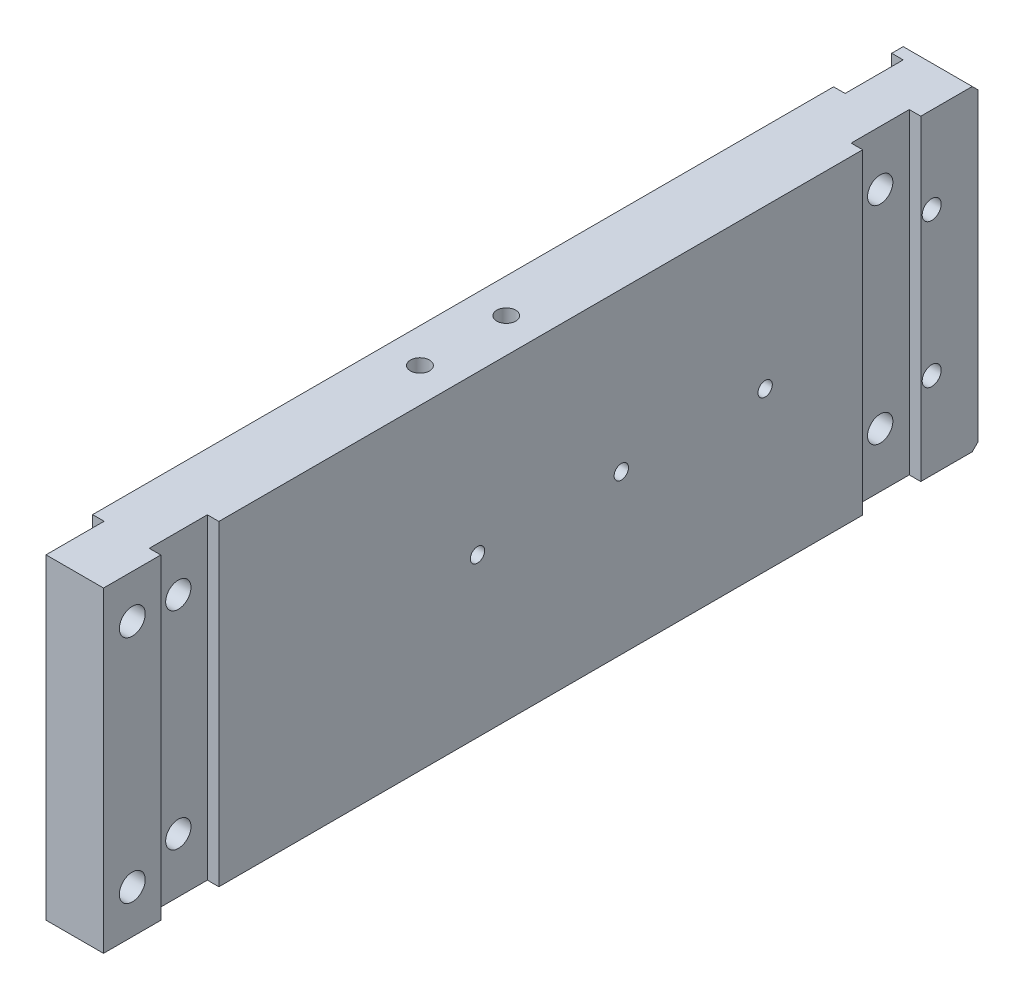
SolidWorks part; units mm, degrees
material "6061铝"
ref_plane "前视基准面" through (0, 0, 0) normal (0, 0, 1) x (1, 0, 0)
ref_plane "上视基准面" through (0, 0, 0) normal (0, 1, 0) x (1, 0, 0)
ref_plane "右视基准面" through (0, 0, 0) normal (1, 0, 0) x (0, 0, -1)
sketch "草图1" plane through (0, 0, 0) normal (1, 0, 0) x (0, 0, -1)
  line L1 (-76, 27.5) -> (76, 27.5)
  line L2 (-76, 27.5) -> (-76, -27.5)
  line L3 (-76, -27.5) -> (76, -27.5)
  line L4 (76, 27.5) -> (76, -27.5)
  line L5 (-76, 27.5) -> (76, -27.5) construction
  line L6 (-76, -27.5) -> (76, 27.5) construction
  point P0 (0, 0)
  dimension "D1" = 55
  dimension "D2" = 152
extrude "凸台-拉伸1" add sketch "草图1" along normal blind 12
sketch "草图2" plane through (12, 0, 0) normal (1, 0, 0) x (0, 0, -1)
  line L0 (-76, 27.5) -> (-76, -27.5) construction
  line L1 (-66.05, 33.3411) -> (-55.95, 33.3411)
  line L2 (-66.05, 33.3411) -> (-66.05, -34.4007)
  line L3 (-66.05, -34.4007) -> (-55.95, -34.4007)
  line L4 (-55.95, 33.3411) -> (-55.95, -34.4007)
  line L5 (-66.05, 33.3411) -> (-55.95, -34.4007) construction
  line L6 (-66.05, -34.4007) -> (-55.95, 33.3411) construction
  point P0 (-61, -0.5298)
  dimension "D1" = 10.1
  dimension "D2" = 15
extrude "切除-拉伸1" cut sketch "草图2" against normal blind 2
sketch "草图3" plane through (0, 0, 0) normal (-1, 0, 0) x (0, 0, 1)
  line L0 (0, 0) -> (-87.8664, 0) construction
  line L2 (-54, 6.025) -> (27, 6.025)
  line L3 (-54, 6.025) -> (-54, -6.025)
  line L4 (-54, -6.025) -> (27, -6.025)
  line L5 (27, 6.025) -> (27, -6.025)
  line L6 (-54, 6.025) -> (27, -6.025) construction
  line L7 (-54, -6.025) -> (27, 6.025) construction
  line L8 (76, 27.5) -> (76, -27.5) construction
  point P2 (-13.5, 0)
  dimension "D1" = 12.05
  dimension "D2" = 81
  dimension "D3" = 49
extrude "切除-拉伸2" cut sketch "草图3" against normal blind 1.5
sketch "草图4" plane through (0, 0, 0) normal (-1, 0, 0) x (0, 0, 1)
  circle A0 centre (-54, 6.025) radius 2
  circle A1 centre (-54, -6.025) radius 2
  circle A2 centre (27, -6.025) radius 2
  circle A3 centre (27, 6.025) radius 2
  dimension "D1" = 4
extrude "切除-拉伸3" cut sketch "草图4" against normal up to surface (1.5 mm away) up to face at (1.5, 0, -13.5)
sketch "草图5" plane through (0, -27.5, 0) normal (0, -1, 0) x (1, 0, 0)
  line L2 (0, 76) -> (2, 76)
  line L3 (0, 76) -> (0, 65.9)
  line L4 (0, 65.9) -> (2, 65.9)
  line L6 (2, 76) -> (2, 65.9)
  dimension "D1" = 2
  dimension "D2" = 10.1
extrude "切除-拉伸4" cut sketch "草图5" against normal blind 110
sketch "草图7" plane through (0, 27.5, 0) normal (0, 1, 0) x (1, 0, 0)
  line L0 (0, 76) -> (0, -65.9) construction
  line L1 (-2, 73) -> (2, 73)
  line L2 (-2, 73) -> (-2, 62.9)
  line L3 (-2, 62.9) -> (2, 62.9)
  line L4 (2, 73) -> (2, 62.9)
  line L5 (-2, 73) -> (2, 62.9) construction
  line L6 (-2, 62.9) -> (2, 73) construction
  line L7 (12, 76) -> (0, 76) construction
  point P0 (0, 67.95)
  dimension "D1" = 10.1
  dimension "D2" = 3
  dimension "D3" = 4
extrude "切除-拉伸5" cut sketch "草图7" against normal blind 120
chamfer "倒角1" distance 1 angle 45 2 edges at (6, -27.5, -76) (6, 27.5, -76)
hole_wizard "M4 螺纹孔1" positions "草图8" profile "草图9" tap size "M4" standard "GB"
sketch "草图8" plane through (0, 27.5, 0) normal (0, 1, 0) x (1, 0, 0)
  line L1 (12, -76) -> (2, -76) construction
  line L2 (12, 75) -> (12, -55.95) construction
  point P0 (6, -15)
  point P2 (6, 0)
  dimension "D1" = 15
  dimension "D2" = 61
  dimension "D3" = 6
cosmetic thread "孔螺蚊线1" parameters "D1"=6, "D2"=4
cosmetic thread "孔螺蚊线2" parameters "D1"=6, "D2"=4
sketch "草图9" plane through (6, 27.5, 15) normal (1, 0, 0) x (0, 0, 1)
  line L0 (0, 0) -> (0, 11.0914)
  line L1 (0, 11.0914) -> (1.65, 10.1)
  line L2 (1.65, 10.1) -> (1.65, 0)
  line L5 (1.65, 0) -> (0, 0)
  line L10 (0, 11.0914) -> (-1.65, 10.1) construction
  line L11 (0, -6.35) -> (0, 107.95) construction
  dimension "螺纹孔钻头直径" = 3.3
  dimension "螺纹孔钻头深度" = 10.1
  dimension "导头角度" = 118
mirror "镜向1" about plane through (0, 0, 0) normal (0, 1, 0) of "M4 螺纹孔1"
hole_wizard "Ø5.0 (5) 直径孔2" positions "草图16" profile "草图17" hole size "Ø5.0" standard "GB"
sketch "草图16" plane through (2, 0, 0) normal (-1, 0, 0) x (0, 0, 1)
  line L0 (0, 0) -> (90.5558, 0) construction
  line L2 (65.9, -27.5) -> (65.9, 27.5) construction
  point P0 (70.9, 12.5)
  point P8 (70.9, -12.5)
  dimension "D1" = 5
  dimension "D2" = 25
sketch "草图17" plane through (2, 12.5, 70.9) normal (0, 1, 0) x (0, 0, 1)
  line L0 (0, 0) -> (0, 7.5022)
  line L1 (0, 7.5022) -> (2.5, 6)
  line L2 (2.5, 6) -> (2.5, 0)
  line L5 (2.5, 0) -> (0, 0)
  line L10 (0, 7.5022) -> (-2.5, 6) construction
  line L11 (0, -6.35) -> (0, 107.95) construction
  dimension "孔直径" = 5
  dimension "孔深度" = 6
  dimension "导头角度" = 118
mirror "镜向2" about plane through (0, 0, 0) normal (0, 0, 1) of "切除-拉伸1"
hole_wizard "打孔尺寸(%根据)内六角圆柱头螺钉的类型1" positions "草图18" profile "草图19" counterbore size "M4" standard "GB" end condition through all
sketch "草图18" plane through (0, 0, 0) normal (-1, 0, 0) x (0, 0, 1)
  point P0 (61, -18)
  point P2 (61, 18)
  point P4 (-61, 18)
  point P6 (-61, -18)
sketch "草图19" plane through (0, -18, 61) normal (0, 1, 0) x (0, 0, 1)
  line L0 (0, 0) -> (0, 12)
  line L1 (0, 12) -> (2.2, 12)
  line L3 (2.2, 12) -> (2.2, 6)
  line L4 (2.2, 6) -> (4, 6)
  line L5 (4, 6) -> (4, 0)
  line L7 (4, 0) -> (0, 0)
  line L11 (0, -6.35) -> (0, 107.95) construction
  dimension "通孔孔直径" = 4.4
  dimension "通孔孔深度" = 12
  dimension "柱形沉头孔直径" = 8
  dimension "柱形沉头孔深度" = 6
hole_wizard "M3 螺纹孔1" positions "草图20" profile "草图22" tap size "M3" standard "GB" end condition through all
sketch "草图20" plane through (0, 0, 0) normal (-1, 0, 0) x (0, 0, 1)
  point P0 (11, 0)
  point P2 (-14, 0)
  point P4 (-39, 0)
sketch "草图22" plane through (0, 0, 11) normal (0, 1, 0) x (0, 0, 1)
  line L0 (0, 0) -> (0, 12)
  line L1 (0, 12) -> (1.25, 12)
  line L2 (1.25, 12) -> (1.25, 0)
  line L5 (1.25, 0) -> (0, 0)
  line L11 (0, -6.35) -> (0, 107.95) construction
  dimension "通孔螺纹孔钻头直径" = 2.5
  dimension "通孔螺纹孔钻头深度" = 12
cosmetic thread "孔螺蚊线3" parameters "D2"=3
cosmetic thread "孔螺蚊线4" parameters "D2"=3
cosmetic thread "孔螺蚊线5" parameters "D2"=3
hole_wizard "M4 螺纹孔2" positions "草图24" profile "草图25" tap size "M4" standard "GB"
sketch "草图24" plane through (0, -27.5, 0) normal (0, -1, 0) x (-1, 0, 0)
  line L0 (-4, 59.926) -> (-8, 59.926) construction
  line L2 (-4, 44.926) -> (-8, 44.926) construction
  point P8 (-6, 59.926)
  point P14 (-6, 44.926)
sketch "草图25" plane through (6, -27.5, -44.926) normal (1, 0, 0) x (0, 0, -1)
  line L0 (0, 0) -> (0, 12.4914)
  line L1 (0, 12.4914) -> (1.65, 11.5)
  line L2 (1.65, 11.5) -> (1.65, 0)
  line L5 (1.65, 0) -> (0, 0)
  line L10 (0, 12.4914) -> (-1.65, 11.5) construction
  line L11 (0, -6.35) -> (0, 107.95) construction
  dimension "螺纹孔钻头直径" = 3.3
  dimension "螺纹孔钻头深度" = 11.5
  dimension "导头角度" = 118
hole_wizard "M4 螺纹孔3" positions "草图27" profile "草图29" tap size "M4" standard "GB" end condition through all
sketch "草图27" plane through (0, 0, 0) normal (-1, 0, 0) x (0, 0, 1)
  point P0 (-67.95, 12.5)
  point P3 (-67.95, -12.5)
sketch "草图29" plane through (0, 12.5, -67.95) normal (0, 1, 0) x (0, 0, 1)
  line L0 (0, 0) -> (0, 12)
  line L1 (0, 12) -> (1.65, 12)
  line L2 (1.65, 12) -> (1.65, 0)
  line L5 (1.65, 0) -> (0, 0)
  line L11 (0, -6.35) -> (0, 107.95) construction
  dimension "通孔螺纹孔钻头直径" = 3.3
  dimension "通孔螺纹孔钻头深度" = 12
cosmetic thread "孔螺蚊线6" parameters "D2"=4
cosmetic thread "孔螺蚊线7" parameters "D2"=4
sketch "草图30" plane through (12, 0, 0) normal (1, 0, 0) x (0, 0, -1)
  circle A0 centre (-71, 20) radius 2.25
  circle A1 centre (-71, -20) radius 2.25
  dimension "D1" = 4.5
extrude "切除-拉伸6" cut sketch "草图30" against normal blind 25
